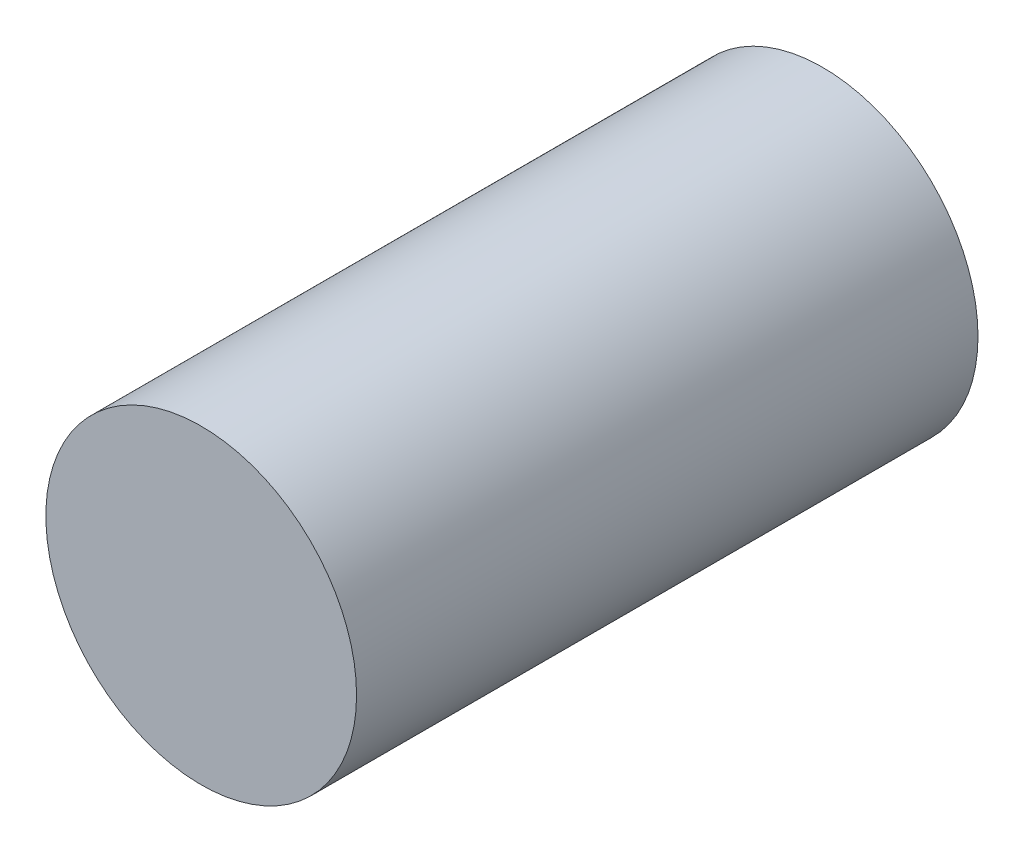
SolidWorks part; units mm, degrees
ref_plane "Front Plane" through (0, 0, 0) normal (0, 0, 1) x (1, 0, 0)
ref_plane "Top Plane" through (0, 0, 0) normal (0, 1, 0) x (1, 0, 0)
ref_plane "Right Plane" through (0, 0, 0) normal (1, 0, 0) x (0, 0, -1)
other "Configuration Table"
sketch "Sketch1" plane through (0, 0, 0) normal (0, 0, 1) x (1, 0, 0)
  circle A0 centre (0, 0) radius 10
  dimension "D1" = 20
extrude "Boss-Extrude1" add sketch "Sketch1" along normal mid plane 40
